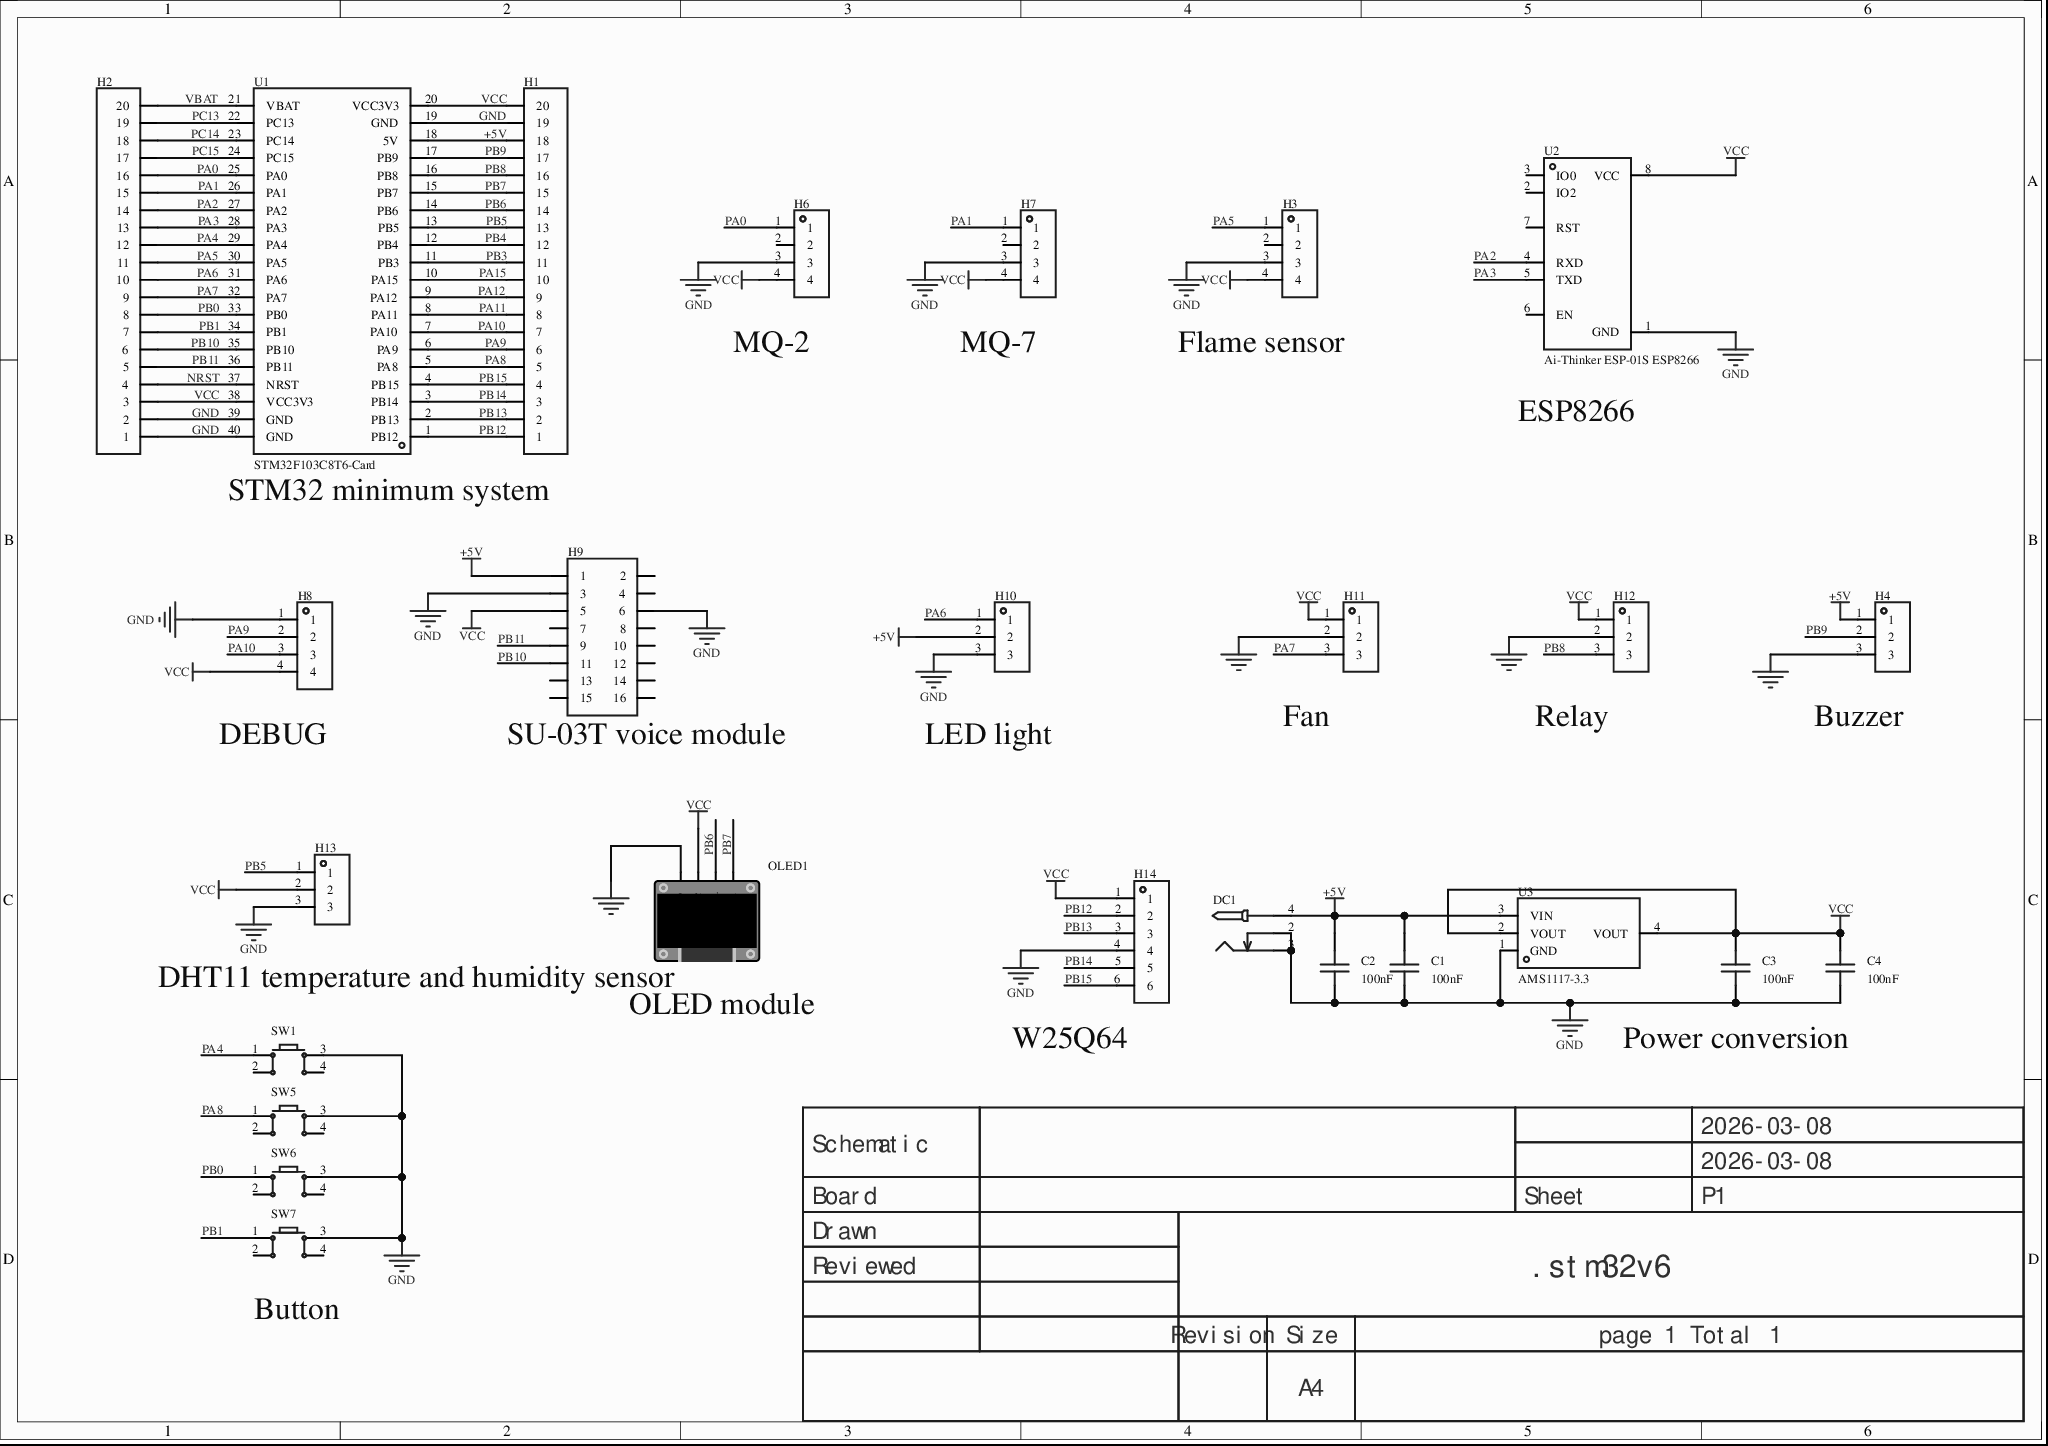
[diagram p0: MISC51915-3.schdoc]
# Altium project MISC51915-2.PrjPcb
1 sheet, 26 parts. Net scope: global (net labels, ports and power ports of the same name join across sheets).
Board file: MISC51915.pcbdoc

## Sheet MISC51915-3.schdoc
size 297 x 209 mm; Version: V1.0; @Project Name: MISC51915; @Page Count: 1; @Update Date: 2026-03-08; @Create Date: 2026-03-08; @Schematic Name: MISC51915; @Page No: 1; @Create Time: 23:22:16; @Update Time: 17:32:40; @Board Name: MISC51915

### Parts
C1  100nF  [C0603]
C2  100nF  [C0603]
C3  100nF  [C0603]
C4  100nF  [C0603]
DC1  (no value)  [DC-2.0]
H1  (no value)  [HDR-TH_20P-P2.54-V-F]
H2  (no value)  [HDR-TH_20P-P2.54-V-F]
H3  (no value)  [HDR-TH_4P-P2.54-V-F]
H4  (no value)  [HDR-TH_3P-P2.54-V-F]
H6  (no value)  [HDR-TH_4P-P2.54-V-F]
H7  (no value)  [HDR-TH_4P-P2.54-V-F]
H8  (no value)  [HDR-TH_4P-P2.54-V-F]
H9  (no value)  [HDR-TH_16P-P2.54-V-M-R2-C8-S2.54]
H10  (no value)  [HDR-TH_3P-P2.54-V-F]
H11  (no value)  [HDR-TH_3P-P2.54-V-F]
H12  (no value)  [HDR-TH_3P-P2.54-V-F]
H13  (no value)  [HDR-TH_3P-P2.54-V-F]
H14  (no value)  [HDR-TH_6P-P2.54-V-F]
OLED1  (no value)  [0.96OLED_4P]
SW1  (no value)  [SW-TH_4P-L6.0-W6.0-P4.50-LS6.5]
SW5  (no value)  [SW-TH_4P-L6.0-W6.0-P4.50-LS6.5]
SW6  (no value)  [SW-TH_4P-L6.0-W6.0-P4.50-LS6.5]
SW7  (no value)  [SW-TH_4P-L6.0-W6.0-P4.50-LS6.5]
U1  STM32F103C8T6-Card  [CONN-TH_L53.3-W22.9_STM32F103C8T6-CARD]
U2  Ai-Thinker ESP-01S ESP8266  [WIFIM-TH_8P-L24.7-W14.4-P2.54]
U3  AMS1117-3.3  [SOT-223-3_L6.5-W3.4-P2.30-LS7.0-BR]

### Nets
+5V: C1.2 C2.2 DC1.4 H1.18 H4.1 H9.1 H10.2 U1.18(5V) U3.3(VIN)
GND: C1.1 C2.1 C3.1 C4.1 DC1.2 DC1.3 H1.19 H2.1 H2.2 H3.3 H4.3 H6.3 H7.3 H8.1 H9.3 H9.6 H10.3 H11.2 H12.2 H13.3 H14.4 OLED1.1(GND) SW1.3 SW5.3 SW6.3 SW7.3 U1.19(GND) U1.39(GND) U1.40(GND) U2.1(GND) U3.1(GND)
VCC: C3.2 C4.2 H1.20 H2.3 H3.4 H6.4 H7.4 H8.4 H9.5 H11.1 H12.1 H13.2 H14.1 OLED1.2(VCC) U1.20(VCC3V3) U1.38(VCC3V3) U2.8(VCC) U3.2(VOUT) U3.4(VOUT)
NRST: H2.4 U1.37(NRST)
PA0: H2.16 H6.1 U1.25(PA0)
PA1: H2.15 H7.1 U1.26(PA1)
PA2: H2.14 U1.27(PA2) U2.4(RXD)
PA3: H2.13 U1.28(PA3) U2.5(TXD)
PA4: H2.12 SW1.1 U1.29(PA4)
PA5: H2.11 H3.1 U1.30(PA5)
PA6: H2.10 H10.1 U1.31(PA6)
PA7: H2.9 H11.3 U1.32(PA7)
PA8: H1.5 SW5.1 U1.5(PA8)
PA9: H1.6 H8.2 U1.6(PA9)
PA10: H1.7 H8.3 U1.7(PA10)
PA11: H1.8 U1.8(PA11)
PA12: H1.9 U1.9(PA12)
PA15: H1.10 U1.10(PA15)
PB0: H2.8 SW6.1 U1.33(PB0)
PB1: H2.7 SW7.1 U1.34(PB1)
PB3: H1.11 U1.11(PB3)
PB4: H1.12 U1.12(PB4)
PB5: H1.13 H13.1 U1.13(PB5)
PB6: H1.14 OLED1.3(SCL) U1.14(PB6)
PB7: H1.15 OLED1.4(SDA) U1.15(PB7)
PB8: H1.16 H12.3 U1.16(PB8)
PB9: H1.17 H4.2 U1.17(PB9)
PB10: H2.6 H9.11 U1.35(PB10)
PB11: H2.5 H9.9 U1.36(PB11)
PB12: H1.1 H14.2 U1.1(PB12)
PB13: H1.2 H14.3 U1.2(PB13)
PB14: H1.3 H14.5 U1.3(PB14)
PB15: H1.4 H14.6 U1.4(PB15)
PC13: H2.19 U1.22(PC13)
PC14: H2.18 U1.23(PC14)
PC15: H2.17 U1.24(PC15)
VBAT: H2.20 U1.21(VBAT)

Not connected (* = marked no-connect by the designer): H3 2; H6 2; H7 2; H9 2 4 7 8 10 12 13 14 15 16; SW1 2 4; SW5 2 4; SW6 2 4; SW7 2 4; U2 2(IO2) 3(IO0) 6(EN) 7(RST)

### Notes on the sheet
- (near H6) MQ-2
- (near H7) MQ-7
- (near H3) Flame sensor
- (near U2) ESP8266
- STM32 minimum system
- (near H8) DEBUG
- (near H9) SU-03T voice module
- (near H10) LED light
- (near H11) Fan
- (near H12) Relay
- (near H4) Buzzer
- DHT11 temperature and humidity sensor
- OLED module
- (near H14) W25Q64
- Power conversion
- (near SW7) Button
- 2026-03-08
- Schematic
- Board
- Sheet
- P1
- Drawn
- Reviewed
- .stm32v6
- Revision
- Size
- A4
- page 1 Total 1

### Library data of the parts
C1-C4 = CAP_0603: Symbol: Capacitance; ConvertToPcb: yes; ModelId: ac125912035d415993ca9572d50418b10819f05c4eef4c71ace90d822a990e87; ModelName: C0603_L1.6-W0.8-H0.8; ModelTransform: 62.992,31.496,0,0,0,0,0,0,0; Device: CAP_0603; AddInBom: yes; Supplier Footprint: 0603; FootprintName: C0603; Value: 100nF
DC1 = DC-005_2.0: Symbol: DC power jack; ConvertToPcb: yes; ModelId: f5f20b8a2308479b936ba3c2698865bb0819f05c4eef4c71ace90d822a990e87; ModelName: DC-IN-TH_DC-5520-1; ModelTransform: 372.05,551.18,582.68,90,0,0,137.8,0,-149.61; Device: DC-005_2.0; AddInBom: yes; Supplier Footprint: 插件; FootprintName: DC-2.0
H1 H2 = HDR-F_2.54_1x20P: ConvertToPcb: yes; ModelId: db7015f7ad9d48b8a3b1188db02e3429; ModelName: HDR-F-2.54_1x20; ModelTransform: 1999.996,100,0,0,0,0,0,0,-118.11; Device: HDR-F_2.54_1x20P; Symbol: HDR-F_2.54_1x20P; AddInBom: yes; SupplierPart: C50984; Supplier Footprint: 插件; FootprintName: HDR-TH_20P-P2.54-V-F
H3 = HDR-F_2.54_1x4P: Symbol: 2.54-1*4P female; 3D Model: d187812051054f85879fcaa51a310d8e0819f05c4eef4c71ace90d822a990e87; 3D Model Transform: 419.6842,98.464,0,0,0,0,0,0,-118.11; ConvertToPcb: yes; Device: HDR-F_2.54_1x4P; Supplier Part: C2718488; Supplier Footprint: 插件; AddInBom: yes; FootprintName: HDR-TH_4P-P2.54-V-F; ModelName: HDR-TH_4P-P2.54-V-F
H4 H10-H13 = HDR-F_2.54_1x3P: Symbol: PM254V-11-03-H85; 3D Model: f3b3cc5aae9641bf9e56fc160cef875b; 3D Model Transform: 299.9994,100,0,0,0,0,0,0,-118.11; ConvertToPcb: yes; ModelName: HDR2.54-F-LI-1X3P; Device: HDR-F_2.54_1x3P; Supplier Part: C541850; Supplier Footprint: 插件; AddInBom: yes; FootprintName: HDR-TH_3P-P2.54-V-F
H6-H8 = HDR-F_2.54_1x4P: Symbol: 2.54-1*4P female; ConvertToPcb: yes; ModelId: d187812051054f85879fcaa51a310d8e0819f05c4eef4c71ace90d822a990e87; ModelTransform: 419.6842,98.464,0,0,0,0,0,0,-118.11; Device: HDR-F_2.54_1x4P; AddInBom: yes; SupplierPart: C2718488; Supplier Footprint: 插件; FootprintName: HDR-TH_4P-P2.54-V-F; ModelName: HDR-TH_4P-P2.54-V-F
H9 = HDR-M_2.54_2x8: Symbol: HDR-M-2.54_2x8; ConvertToPcb: yes; ModelId: 4229ed04564d49dfa51d40f734d422b60819f05c4eef4c71ace90d822a990e87; ModelName: HDR2.54-M-LI-2X8P; ModelTransform: 799.99844,200,0,0,0,0,0,0,-118.11; Device: HDR-M_2.54_2x8; AddInBom: yes; SupplierPart: C68234; Supplier Footprint: 插件,P=2.54mm; FootprintName: HDR-TH_16P-P2.54-V-M-R2-C8-S2.54
H14 = HDR-F_2.54_1x6P: Symbol: Header-Female-2.54_1x6; ConvertToPcb: yes; ModelId: 0f5bcf94dcda47d085f24cdca1696fe9; ModelTransform: 619.684,94.488,0,0,0,0,0,0,-125.984; Device: HDR-F_2.54_1x6P; AddInBom: yes; SupplierPart: C40877; Supplier Footprint: 插件; FootprintName: HDR-TH_6P-P2.54-V-F; ModelName: HDR-TH_6P-P2.54-V-F
OLED1 = 0.96OLED模块_4P: Device: 0.96OLED module_4P; ConvertToPcb: yes; ModelId: 79c000fdb68d45a296c2e9bedf4f9055; ModelTransform: 1393.69792,1318.895,0,0,0,0,0,-560.079,-137.795; Symbol: 0.96OLED module_4P; AddInBom: yes; FootprintName: 0.96OLED_4P; Supplier Footprint: 插件; ModelName: 0.96OLED_4P
SW1 = Key_TH_6x6x6: 触点电流:50mA;额定电压(DC):12V;绝缘电阻:100MΩ;电路结构:单刀单掷;安装方式:直插;按钮形状:圆形按钮;按钮/盖帽颜色:黑色;作用力:260gf@±30gf;工作温度:-25℃~+70℃;引脚样式:PC引脚;开关长度:6mm;开关宽度:6mm;开关高度:6mm;带支架:否;; Symbol: Tact switch; 3D Model: 20eee248bc684ccd8cbdbb1d0d91ec6f; 3D Model Transform: 236.22,323.03,0,90,0,0,0,0,-137.795; ConvertToPcb: yes; ModelName: SW-TH_4P-L6.0-W6.0-H5.0-LS6.5-P4.50; Device: Key_TH_6x6x6; Supplier Part: C2837516; Supplier Footprint: 插件; AddInBom: yes; FootprintName: SW-TH_4P-L6.0-W6.0-P4.50-LS6.5
SW5-SW7 = Key_TH_6x6x6: 触点电流:50mA;额定电压(DC):12V;绝缘电阻:100MΩ;电路结构:单刀单掷;安装方式:直插;按钮形状:圆形按钮;按钮/盖帽颜色:黑色;作用力:260gf@±30gf;工作温度:-25℃~+70℃;引脚样式:PC引脚;开关长度:6mm;开关宽度:6mm;开关高度:6mm;带支架:否;; Symbol: Tact switch; ConvertToPcb: yes; ModelId: 20eee248bc684ccd8cbdbb1d0d91ec6f; ModelName: SW-TH_4P-L6.0-W6.0-H5.0-LS6.5-P4.50; ModelTransform: 236.22,323.03,0,90,0,0,0,0,-137.795; Device: Key_TH_6x6x6; AddInBom: yes; SupplierPart: C2837516; Supplier Footprint: 插件; FootprintName: SW-TH_4P-L6.0-W6.0-P4.50-LS6.5
U1 = STM32F103C8T6-Card: AddInBom: yes; Symbol: STM32F103C8T6-CARD; Device: STM32F103C8T6-Card; LCSC Part Name: STM32F103C8T6-Card; SupplierPart: C9900077949; ManufacturerPart: STM32F103C8T6-Card; Supplier Footprint: 插件; Supplier: LCSC; ConvertToPcb: yes; FootprintName: CONN-TH_L53.3-W22.9_STM32F103C8T6-CARD
U2 = Ai-Thinker ESP-01S ESP8266: Manufacturer: Ai-Thinker(安信可); AddInBom: yes; ModelId: 9453774c1eaa4779b246df5901e962460819f05c4eef4c71ace90d822a990e87; ModelName: WIFIM-TH_8P-L24.7-W14.4-H2.8-P2.54; ModelTransform: 972.43904,566.928,0,0,0,0,377.167,-3.936,-118.11; Symbol: AI-THINKER ESP-01S ESP8266; Device: Ai-Thinker ESP-01S ESP8266; LCSC Part Name: Ai-Thinker ESP-01S ESP8266; SupplierPart: C17606792; ManufacturerPart: Ai-Thinker ESP-01S ESP8266; Supplier Footprint: -; JLCPCB Part Class: Extended Part; Datasheet: https://item.szlcsc.com/datasheet/Ai-Thinker%2520ESP-01S%2520ESP8266/18736031.html; Supplier: LCSC; ConvertToPcb: yes; FootprintName: WIFIM-TH_8P-L24.7-W14.4-P2.54
U3 = AMS1117-3.3_C6186: Output type: fixed; operating voltage: -; output voltage: 3.3V; output current: 1A; ripple rejection (PSRR): 72dB@(120Hz); output polarity: positive;; Manufacturer: AMS; AddInBom: yes; ModelId: 925194bf9823436183a3e0b978a8d076; ModelName: SOT-223-4P_L6.5-W3.5-H1.6-LS7.0-P2.30; ModelTransform: 279.89794,255.905,0,180,0,0,-3.9385,-0.0005,0; Voltage Dropout: 1.3V@(800mA); Number of Outputs: 1; Symbol: AMS1117-3.3; Device: AMS1117-3.3_C6186; LCSC Part Name: 输出3.3V 1A; SupplierPart: C6186; ManufacturerPart: AMS1117-3.3; Supplier Footprint: SOT-223; Datasheet: https://atta.szlcsc.com/upload/public/pdf/source/20180727/C6186_7A095716F0823C02F1997A905E26C086.pdf; Supplier: LCSC; ConvertToPcb: yes; FootprintName: SOT-223-3_L6.5-W3.4-P2.30-LS7.0-BR; Output Type: Fixed; Voltage - Supply: -; Output Voltage: 3.3V; Output Current: 1A; Power Supply Rejection Ratio (PSRR): 72dB@(120Hz); standby current: -; Noise: -; Features: Overcurrent protection (OCP); thermal shutdown (TSD); Operating Temperature: -; Output Configuration: Positive